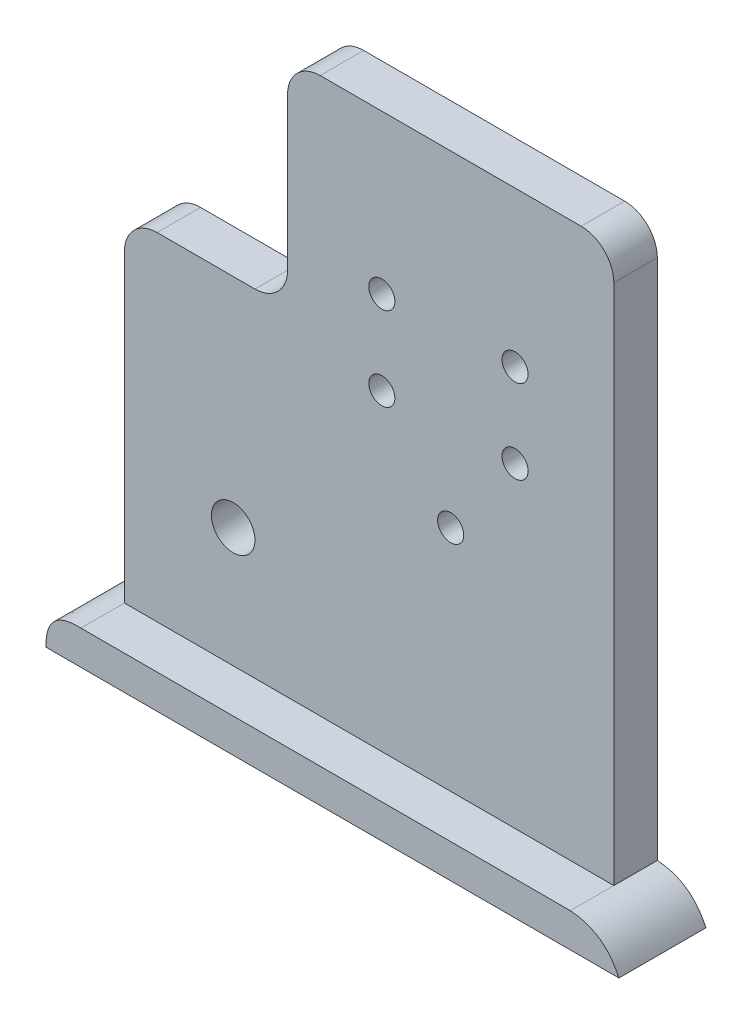
from build123d import *

# Parameters (mm, degrees)
SKETCH1_W           = 600
SKETCH1_H           = 600
BOSS_EXTRUDE1_DEPTH = 40
SKETCH2_R           = 20
CUT_EXTRUDE1_DEPTH  = 40
SKETCH3_R           = 12
CUT_EXTRUDE2_DEPTH  = 60
SKETCH4_R           = 12
CUT_EXTRUDE3_DEPTH  = 90
SKETCH5_W           = 150
SKETCH5_H           = 600
CUT_EXTRUDE4_DEPTH  = 100
SKETCH6_W           = 150
SKETCH6_H           = 200
CUT_EXTRUDE5_DEPTH  = 100
SKETCH7_W           = 450
SKETCH7_H           = 90
CUT_EXTRUDE6_DEPTH  = 100
SKETCH9_R           = 12
CUT_EXTRUDE7_DEPTH  = 50
FILLET1_R           = 30
BOSS_EXTRUDE2_DEPTH = 80


with BuildPart() as part:
    # Sketch1 → Boss-Extrude1 (new body)
    with BuildSketch(Plane.XY):
        Rectangle(SKETCH1_W, SKETCH1_H)
    extrude(amount=BOSS_EXTRUDE1_DEPTH)

    # Sketch2 → Cut-Extrude1 (cut)
    with BuildSketch(Plane.XY.offset(40)):
        with Locations((-200, -100)):
            Circle(SKETCH2_R)
    extrude(amount=-CUT_EXTRUDE1_DEPTH, mode=Mode.SUBTRACT)

    # Sketch3 → Cut-Extrude2 (cut)
    with BuildSketch(Plane.XY.offset(40)):
        Circle(SKETCH3_R)
    extrude(amount=-CUT_EXTRUDE2_DEPTH, mode=Mode.SUBTRACT)

    # Sketch4 → Cut-Extrude3 (cut)
    with BuildSketch(Plane.XY.offset(40)):
        with Locations((-63.335275248, 77.386322495)):
            Circle(SKETCH4_R)
        with Locations((59.168411159, 80.616990275)):
            Circle(SKETCH4_R)
    extrude(amount=-CUT_EXTRUDE3_DEPTH, mode=Mode.SUBTRACT)

    # Sketch5 → Cut-Extrude4 (cut)
    with BuildSketch(Plane.XY.offset(40)):
        with Locations((225, 0)):
            Rectangle(SKETCH5_W, SKETCH5_H)
    extrude(amount=-CUT_EXTRUDE4_DEPTH, mode=Mode.SUBTRACT)

    # Sketch6 → Cut-Extrude5 (cut)
    with BuildSketch(Plane.XY.offset(40)):
        with Locations((-225, 200)):
            Rectangle(SKETCH6_W, SKETCH6_H)
    extrude(amount=-CUT_EXTRUDE5_DEPTH, mode=Mode.SUBTRACT)

    # Sketch7 → Cut-Extrude6 (cut)
    with BuildSketch(Plane.XY.offset(40)):
        with Locations((-75, -255)):
            Rectangle(SKETCH7_W, SKETCH7_H)
    extrude(amount=-CUT_EXTRUDE6_DEPTH, mode=Mode.SUBTRACT)

    # Sketch9 → Cut-Extrude7 (cut)
    with BuildSketch(Plane.XY.offset(40)):
        with Locations((-63.335275248, 154.386322495)):
            Circle(SKETCH9_R)
        with Locations((59.168411159, 157.616990275)):
            Circle(SKETCH9_R)
    extrude(amount=-CUT_EXTRUDE7_DEPTH, mode=Mode.SUBTRACT)

    # Fillet1
    fillet1_edges = [part.edges().sort_by_distance(p)[0] for p in [
        (150, 300, 20),
        (-300, 100, 20),
        (-150, 300, 20),
        (-150, 100, 20),
    ]]
    fillet(fillet1_edges, radius=FILLET1_R)

    # Sketch10 → Boss-Extrude2 (add)
    with BuildSketch(Plane(origin=(0, 0, 0), x_dir=(-1, 0, 0), z_dir=(0, 0, -1))):
        with BuildLine():
            Line((-150, -210), (300, -210))
            add(Edge.make_bspline(
                [(300, -210), (333.145645994, -208.556298113), (332.053728057, -241.264865933)],
                knots=[0, 0, 0, 1, 1, 1], degree=2))
            Line((332.053728057, -241.264865933), (-194.702453995, -241.264865933))
            add(Edge.make_bspline(
                [(-150, -210), (-181.312836573, -212.059215881), (-194.702453995, -241.264865933)],
                knots=[0, 0, 0, 1, 1, 1], degree=2))
        make_face()
    extrude(amount=-BOSS_EXTRUDE2_DEPTH)


solid = part.part
